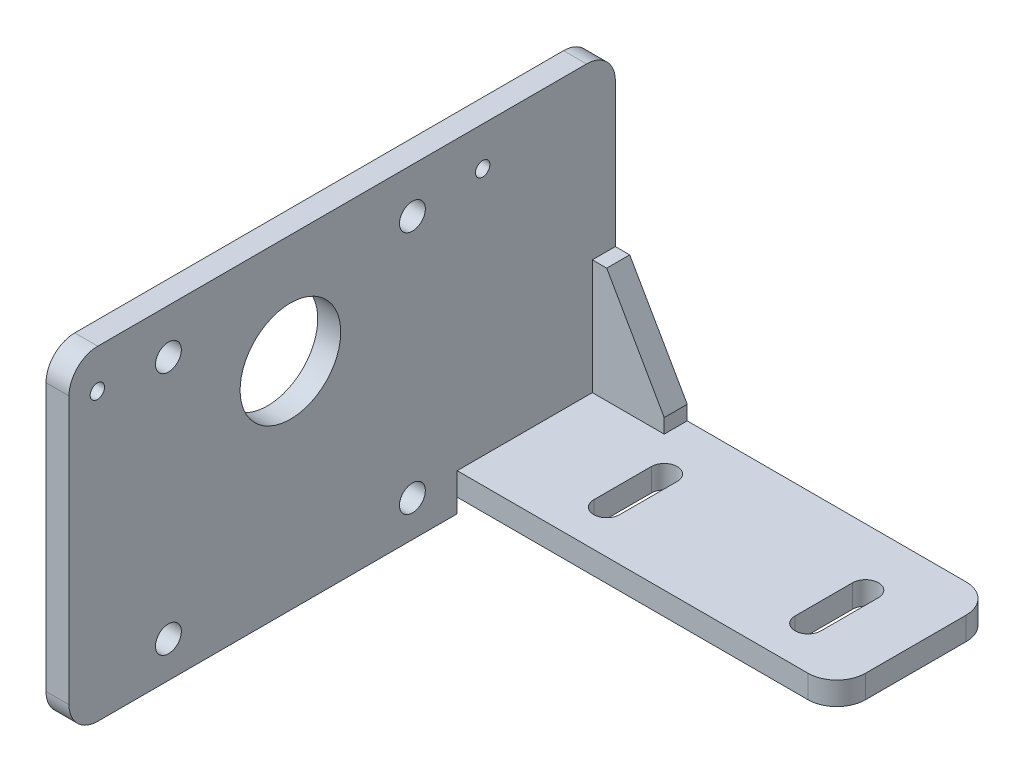
from build123d import *

# Parameters (mm, degrees)
EXTRUDE_1_DEPTH     = 95
SKETCH_2_R          = 4.5
CUT_EXTRUDE_1_DEPTH = 10
EXTRUDE_1_2_DEPTH   = 8
SKETCH_5_R          = 4.5
SKETCH_5_R_2        = 17.5
CUT_EXTRUDE_2_DEPTH = 196.225510628
FILLET_1_R          = 10
CUT_EXTRUDE_4_DEPTH = 10
SKETCH_8_W          = 132
SKETCH_8_H          = 163.82032184
CUT_EXTRUDE_5_DEPTH = 10
FILLET_2_R          = 10
SKETCH_9_W          = 8
SKETCH_9_H          = 135
EXTRUDE_2_DEPTH     = 5
FILLET_3_R          = 10
SKETCH_10_R         = 2.5
CUT_EXTRUDE_6_DEPTH = 10


with BuildPart() as part:
    # 草图1 → Extrude 1 (new, symmetric)
    with BuildSketch(Plane.XY):
        Polygon((0, 108), (0, 0), (140, 0), (140, 8), (8, 8), (8, 108), align=None)
    extrude(amount=EXTRUDE_1_DEPTH, both=True)

    # 草图2 → 切除-拉伸1 (cut)
    with BuildSketch(Plane(origin=(0, 8, 0), x_dir=(1, 0, 0), z_dir=(0, 1, 0))):
        with Locations(Location((115, 65, 0), (0, 0, 270))):
            Circle(SKETCH_2_R)
        with Locations(Location((45, 65, 0), (0, 0, 270))):
            Circle(SKETCH_2_R)
        with Locations(Location((115, -65, 0), (0, 0, 270))):
            Circle(SKETCH_2_R)
        with Locations(Location((45, -65, 0), (0, 0, 270))):
            Circle(SKETCH_2_R)
    extrude(amount=-CUT_EXTRUDE_1_DEPTH, mode=Mode.SUBTRACT)

    # 草图5 → 切除-拉伸2 (cut, through all)
    with BuildSketch(Plane(origin=(8, 0, 0), x_dir=(0, 0, -1), z_dir=(1, 0, 0))):
        with Locations(Location((-60.426406871, 92.426406871, 0), (0, 0, 90))):
            Circle(SKETCH_5_R)
        with Locations(Location((-60.426406871, 7.573593129, 0), (0, 0, 90))):
            Circle(SKETCH_5_R)
        with Locations(Location((24.426406871, 7.573593129, 0), (0, 0, 90))):
            Circle(SKETCH_5_R)
        with Locations(Location((24.426406871, 92.426406871, 0), (0, 0, 90))):
            Circle(SKETCH_5_R)
        with Locations(Location((-18, 70, 0), (0, 0, 90))):
            Circle(SKETCH_5_R_2)
    extrude(amount=-CUT_EXTRUDE_2_DEPTH, mode=Mode.SUBTRACT)

    # 圆角1
    fillet_1_edges = [part.edges().sort_by_distance(p)[0] for p in [
        (4, 108, -95),
        (4, 108, 95),
        (140, 4, 95),
        (140, 4, -95),
    ]]
    fillet(fillet_1_edges, radius=FILLET_1_R)

    # 草图7 → 切除-拉伸4 (cut)
    with BuildSketch(Plane(origin=(0, 8, 0), x_dir=(1, 0, 0), z_dir=(0, 1, 0))):
        with BuildLine():
            Line((40.5, 55), (40.5, 75))
            ThreePointArc((40.5, 75), (45, 79.5), (49.5, 75))
            Line((49.5, 75), (49.5, 55))
            ThreePointArc((49.5, 55), (45, 50.5), (40.5, 55))
        make_face()
        with BuildLine():
            Line((110.5, 55), (110.5, 75))
            ThreePointArc((110.5, 75), (115, 79.5), (119.5, 75))
            Line((119.5, 75), (119.5, 55))
            ThreePointArc((119.5, 55), (115, 50.5), (110.5, 55))
        make_face()
        with BuildLine():
            Line((110.5, -75), (110.5, -55))
            ThreePointArc((110.5, -55), (115, -50.5), (119.5, -55))
            Line((119.5, -55), (119.5, -75))
            ThreePointArc((119.5, -75), (115, -79.5), (110.5, -75))
        make_face()
        with BuildLine():
            Line((40.5, -75), (40.5, -55))
            ThreePointArc((40.5, -55), (45, -50.5), (49.5, -55))
            Line((49.5, -55), (49.5, -75))
            ThreePointArc((49.5, -75), (45, -79.5), (40.5, -75))
        make_face()
    extrude(amount=-CUT_EXTRUDE_4_DEPTH, mode=Mode.SUBTRACT)

    # 草图8 → 切除-拉伸5 (cut)
    with BuildSketch(Plane(origin=(0, 8, 0), x_dir=(1, 0, 0), z_dir=(0, 1, 0))):
        with Locations((74, -41.91016092)):
            Rectangle(SKETCH_8_W, SKETCH_8_H)
    extrude(amount=-CUT_EXTRUDE_5_DEPTH, mode=Mode.SUBTRACT)

    # 圆角2
    fillet_2_edges = [part.edges().sort_by_distance(p)[0] for p in [
        (140, 4, -40),
    ]]
    fillet(fillet_2_edges, radius=FILLET_2_R)

    # 草图9 → 凸台-拉伸2 (add)
    with BuildSketch(Plane.XZ):
        with Locations((4, 27.5)):
            Rectangle(SKETCH_9_W, SKETCH_9_H)
    extrude(amount=EXTRUDE_2_DEPTH)

    # 圆角3
    fillet_3_edges = [part.edges().sort_by_distance(p)[0] for p in [
        (4, -5, 95),
    ]]
    fillet(fillet_3_edges, radius=FILLET_3_R)

    # 草图10 → 切除-拉伸6 (cut)
    with BuildSketch(Plane(origin=(8, 0, 0), x_dir=(0, 0, -1), z_dir=(1, 0, 0))):
        with Locations(Location((-85.142306872, 94.5, 0), (0, 0, 90))):
            Circle(SKETCH_10_R)
        with Locations(Location((48.857693128, 94.5, 0), (0, 0, 90))):
            Circle(SKETCH_10_R)
    extrude(amount=-CUT_EXTRUDE_6_DEPTH, mode=Mode.SUBTRACT)


with BuildPart() as body_2:
    # 草图4 → Extrude 1 2 (new body)
    with BuildSketch(Plane.XY.offset(95)):
        Polygon((8, 48), (13, 48), (33, 13), (33, 8), (8, 8), align=None)
    extrude(amount=-EXTRUDE_1_2_DEPTH)


with BuildPart() as body_3:
    # 镜向2: mirrored copy
    add(body_2.part.mirror(Plane.XY))


solid = Compound([part.part, body_3.part])
